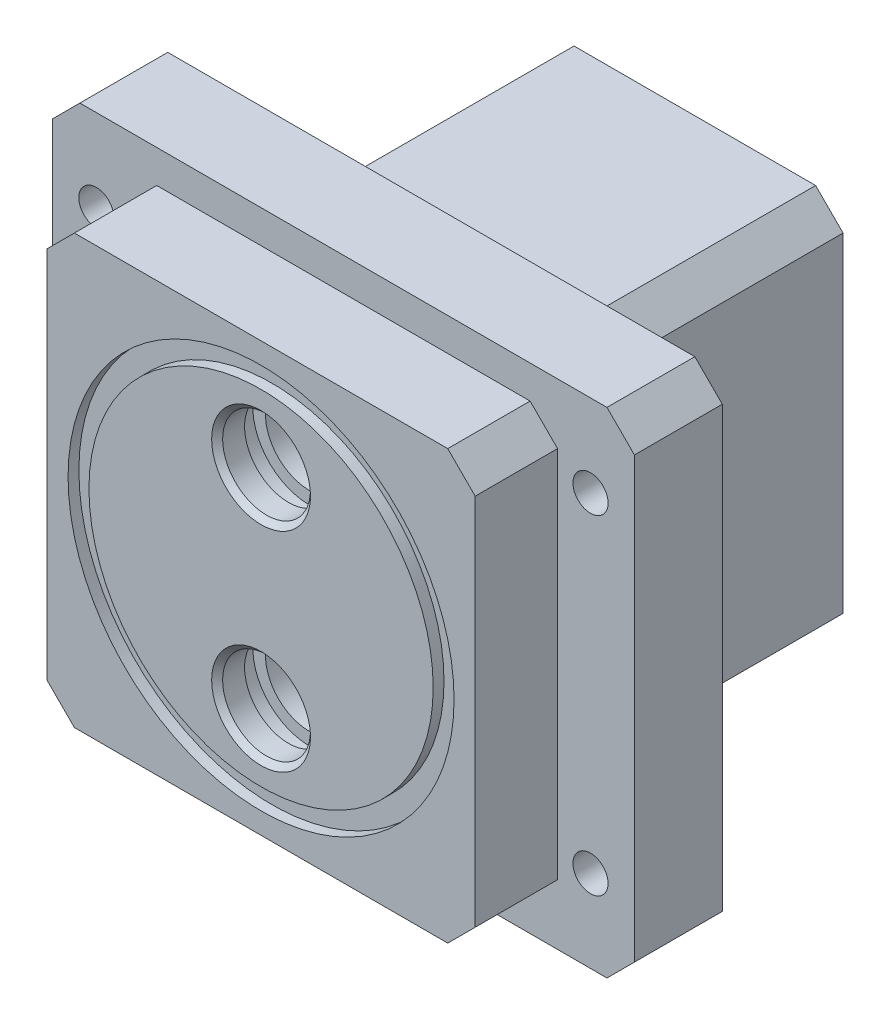
SolidWorks part; units mm, degrees
material "Q235-A"
ref_plane "Front Plane" through (0, 0, 0) normal (0, 0, 1) x (1, 0, 0)
ref_plane "Top Plane" through (0, 0, 0) normal (0, 1, 0) x (1, 0, 0)
ref_plane "Right Plane" through (0, 0, 0) normal (1, 0, 0) x (0, 0, -1)
sketch "Sketch1" plane through (0, 0, 0) normal (0, 0, 1) x (1, 0, 0)
  line L1 (-27, -35) -> (27, -35)
  line L2 (-27, -35) -> (-27, 35)
  line L3 (-27, 35) -> (27, 35)
  line L4 (27, -35) -> (27, 35)
  line L5 (-27, -35) -> (27, 35) construction
  line L6 (-27, 35) -> (27, -35) construction
  point P0 (0, 0)
  dimension "D1" = 54
  dimension "D2" = 70
extrude "Boss-Extrude1" add sketch "Sketch1" along normal blind 48
sketch "Sketch2" plane through (0, 0, 48) normal (0, 0, 1) x (1, 0, 0)
  line L1 (53, 45) -> (-53, 45)
  line L2 (53, 45) -> (53, -45)
  line L3 (53, -45) -> (-53, -45)
  line L4 (-53, 45) -> (-53, -45)
  line L5 (53, 45) -> (-53, -45) construction
  line L6 (53, -45) -> (-53, 45) construction
  point P0 (0, 0)
  dimension "D1" = 106
  dimension "D2" = 90
extrude "Boss-Extrude2" add sketch "Sketch2" along normal blind 16
sketch "Sketch3" plane through (0, 0, 64) normal (0, 0, 1) x (1, 0, 0)
  line L1 (39, 39) -> (-39, 39)
  line L2 (39, 39) -> (39, -39)
  line L3 (39, -39) -> (-39, -39)
  line L4 (-39, 39) -> (-39, -39)
  line L5 (39, 39) -> (-39, -39) construction
  line L6 (39, -39) -> (-39, 39) construction
  point P0 (0, 0)
  dimension "D1" = 78
  dimension "D2" = 78
extrude "Boss-Extrude3" add sketch "Sketch3" along normal blind 15
chamfer "Chamfer1" distance 5 angle 45 12 edges at (-27, 35, 24) (-53, 45, 56) (-39, 39, 71.5) (-53, -45, 56) (-27, -35, 24) (-39, -39, 71.5) (39, -39, 71.5) (39, 39, 71.5) (53, 45, 56) (53, -45, 56) (27, 35, 24) (27, -35, 24)
sketch "Sketch4" plane through (0, 0, 79) normal (0, 0, 1) x (1, 0, 0)
  circle A0 centre (0, 0) radius 35.15
  circle A1 centre (0, 0) radius 31.35
extrude "Cut-Extrude1" cut sketch "Sketch4" against normal blind 1.97
sketch "Sketch5" plane through (0, 0, 79) normal (0, 0, 1) x (1, 0, 0)
  line L0 (0, 19) -> (0, -19)
  point P5 (0, 0)
hole_wizard "Hole1" positions "Sketch6" profile "Sketch7" legacy end condition through all
sketch "Sketch6" plane through (0, 0, 79) normal (0, 0, 1) x (1, 0, 0)
  point P0 (0, -19)
  point P3 (0, 19)
sketch "Sketch7" plane through (0, -19, 79) normal (1, 0, 0) x (0, -1, 0)
  line L0 (0, 0) -> (0, 79)
  line L1 (0, 79) -> (8, 79)
  line L2 (8, 79) -> (8, 0)
  line L3 (8, 0) -> (0, 0)
  line L4 (0, 110) -> (0, -10) construction
  dimension "直径" = 16
  dimension "深度" = 79
hole_wizard "Hole2" positions "Sketch8" profile "Sketch9" legacy
sketch "Sketch8" plane through (0, 0, 0) normal (0, 0, -1) x (-1, 0, 0)
  point P0 (0, 19)
  point P3 (0, -19)
sketch "Sketch9" plane through (0, 19, 0) normal (1, 0, 0) x (0, 1, 0)
  line L0 (0, 0) -> (0, 63)
  line L1 (0, 63) -> (11, 63)
  line L2 (11, 63) -> (11, 0)
  line L3 (11, 0) -> (0, 0)
  line L4 (0, 110) -> (0, -10) construction
  dimension "直径" = 22
  dimension "深度" = 63
chamfer "Chamfer2" distance 1 angle 45 4 edges at (8, -19, 79) (8, 19, 79) (-11, 19, 0) (-11, -19, 0)
sketch "Sketch10" plane through (0, 0, 0) normal (0, 0, -1) x (-1, 0, 0)
  line L1 (20, 19) -> (-20, 19)
  line L2 (20, 19) -> (20, -19)
  line L3 (20, -19) -> (-20, -19)
  line L4 (-20, 19) -> (-20, -19)
  line L5 (20, 19) -> (-20, -19) construction
  line L6 (20, -19) -> (-20, 19) construction
  point P0 (0, 0)
  dimension "D1" = 38
  dimension "D2" = 40
hole_wizard "M5 Tapped Hole1" positions "Sketch11" profile "Sketch12" tap size "M5" standard "GB"
sketch "Sketch11" plane through (0, 0, 0) normal (0, 0, -1) x (-1, 0, 0)
  point P0 (20, -19)
  point P3 (20, 19)
  point P6 (-20, 19)
  point P9 (-20, -19)
sketch "Sketch12" plane through (-20, -19, 0) normal (1, 0, 0) x (0, 1, 0)
  line L0 (0, 0) -> (0, 11.2618)
  line L1 (0, 11.2618) -> (2.1, 10)
  line L2 (2.1, 10) -> (2.1, 0)
  line L5 (2.1, 0) -> (0, 0)
  line L10 (0, 11.2618) -> (-2.1, 10) construction
  line L11 (0, -6.35) -> (0, 107.95) construction
  dimension "螺纹孔钻头直径" = 4.2
  dimension "螺纹孔钻头深度" = 10
  dimension "导头角度" = 118
cosmetic thread "Cosmetic Thread1" parameters "D1"=10, "D2"=5
cosmetic thread "Cosmetic Thread2" parameters "D1"=10, "D2"=5
cosmetic thread "Cosmetic Thread3" parameters "D1"=10, "D2"=5
cosmetic thread "Cosmetic Thread4" parameters "D1"=10, "D2"=5
sketch "Sketch13" plane through (0, 0, 48) normal (0, 0, -1) x (-1, 0, 0)
  line L1 (45, 30) -> (-45, 30)
  line L2 (45, 30) -> (45, -30)
  line L3 (45, -30) -> (-45, -30)
  line L4 (-45, 30) -> (-45, -30)
  line L5 (45, 30) -> (-45, -30) construction
  line L6 (45, -30) -> (-45, 30) construction
  point P0 (0, 0)
  dimension "D1" = 60
  dimension "D2" = 90
hole_wizard "Hole3" positions "Sketch14" profile "Sketch15" legacy end condition through all
sketch "Sketch14" plane through (0, 0, 48) normal (0, 0, -1) x (-1, 0, 0)
  point P0 (45, -30)
  point P3 (45, 30)
  point P6 (-45, 30)
  point P9 (-45, -30)
sketch "Sketch15" plane through (-45, -30, 48) normal (1, 0, 0) x (0, 1, 0)
  line L0 (0, 0) -> (0, 31)
  line L1 (0, 31) -> (3.2, 31)
  line L2 (3.2, 31) -> (3.2, 9)
  line L3 (3.2, 9) -> (5.5, 9)
  line L4 (5.5, 9) -> (5.5, 0)
  line L5 (5.5, 0) -> (0, 0)
  line L6 (0, 110) -> (0, -10) construction
  dimension "直径" = 6.4
  dimension "深度" = 31
  dimension "柱坑直径" = 11
  dimension "柱坑深度" = 9
ref_plane "Plane1" through (0, 0, 74) normal (0, 0, 1) x (1, 0, 0)
sketch "Sketch16" plane through (0, 0, 74) normal (0, 0, 1) x (1, 0, 0)
  circle A0 centre (0, 19) radius 10.3
  circle A1 centre (0, -19) radius 10.3
extrude "Cut-Extrude2" cut sketch "Sketch16" against normal blind 3.8
